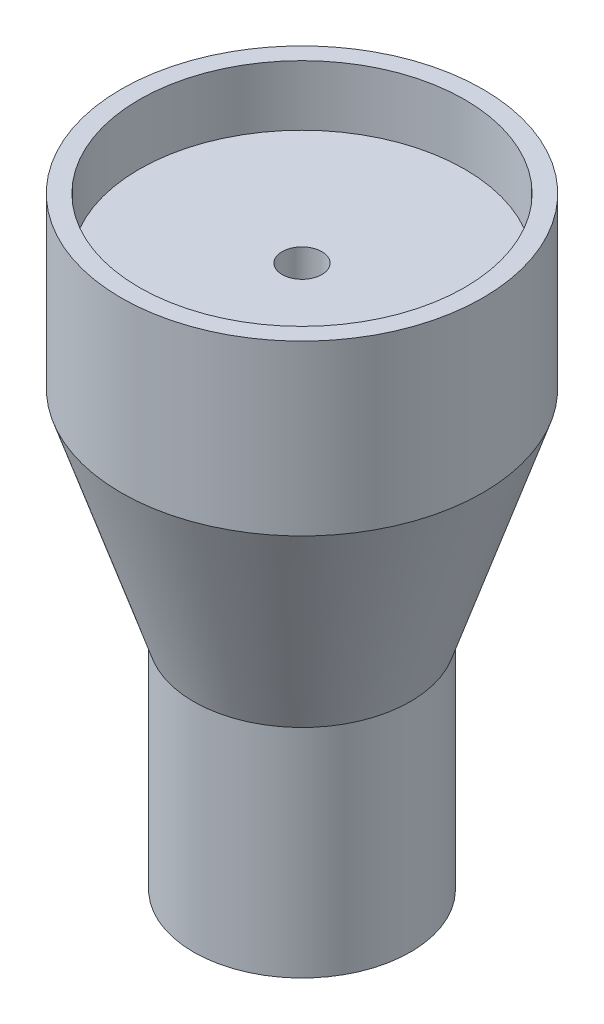
SolidWorks part; units mm, degrees
material "6061 Alloy"
ref_plane "Front Plane" through (0, 0, 0) normal (0, 0, 1) x (1, 0, 0)
ref_plane "Top Plane" through (0, 0, 0) normal (0, 1, 0) x (1, 0, 0)
ref_plane "Right Plane" through (0, 0, 0) normal (1, 0, 0) x (0, 0, -1)
sketch "Sketch1" plane through (0, 0, 0) normal (0, 0, 1) x (1, 0, 0)
  line L0 (0, 0) -> (0, -5.3422) construction
  line L1 (0, 0) -> (-9, 0)
  line L2 (-15, 36) -> (-15, 50)
  line L3 (-15, 50) -> (-13.5, 50)
  line L4 (-13.5, 50) -> (-13.5, 45)
  line L5 (-13.5, 45) -> (0, 45)
  line L6 (0, 45) -> (0, 0)
  line L7 (-15, 36) -> (-9, 18)
  line L8 (-9, 18) -> (-9, 0)
  dimension "D1" = 30
  dimension "D2" = 1.5
  dimension "D3" = 18
  dimension "D4" = 5
  dimension "D5" = 50
  dimension "D6" = 18
  dimension "D7" = 14
revolve "Revolve1" add sketch "Sketch1" angle 360 about L0
hole_wizard "M10x1.0 Tapped Hole1" positions "Sketch2" profile "Sketch3" tap size "M10x1.0" standard "GB"
sketch "Sketch2" plane through (0, 0, 0) normal (0, -1, 0) x (-1, 0, 0)
  point P0 (0, 0)
sketch "Sketch3" plane through (0, 0, 0) normal (1, 0, 0) x (0, 0, -1)
  line L0 (0, 0) -> (0, 30.7039)
  line L1 (0, 30.7039) -> (4.5, 28)
  line L2 (4.5, 28) -> (4.5, 0)
  line L5 (4.5, 0) -> (0, 0)
  line L10 (0, 30.7039) -> (-4.5, 28) construction
  line L11 (0, -6.35) -> (0, 107.95) construction
  dimension "螺纹孔钻头直径" = 9
  dimension "螺纹孔钻头深度" = 28
  dimension "导头角度" = 118
cosmetic thread "Hole Cosmetic Thread1" parameters "D1"=25, "D2"=10
hole_wizard "M4 Tapped Hole1" positions "Sketch4" profile "Sketch5" tap size "M4" standard "GB"
sketch "Sketch4" plane through (0, 45, 0) normal (0, 1, 0) x (1, 0, 0)
  point P0 (0, 0)
sketch "Sketch5" plane through (0, 45, 0) normal (1, 0, 0) x (0, 0, 1)
  line L0 (0, 0) -> (0, 11.0914)
  line L1 (0, 11.0914) -> (1.65, 10.1)
  line L2 (1.65, 10.1) -> (1.65, 0)
  line L5 (1.65, 0) -> (0, 0)
  line L10 (0, 11.0914) -> (-1.65, 10.1) construction
  line L11 (0, -6.35) -> (0, 107.95) construction
  dimension "螺纹孔钻头直径" = 3.3
  dimension "螺纹孔钻头深度" = 10.1
  dimension "导头角度" = 118
cosmetic thread "Hole Cosmetic Thread2" parameters "D1"=8, "D2"=4
